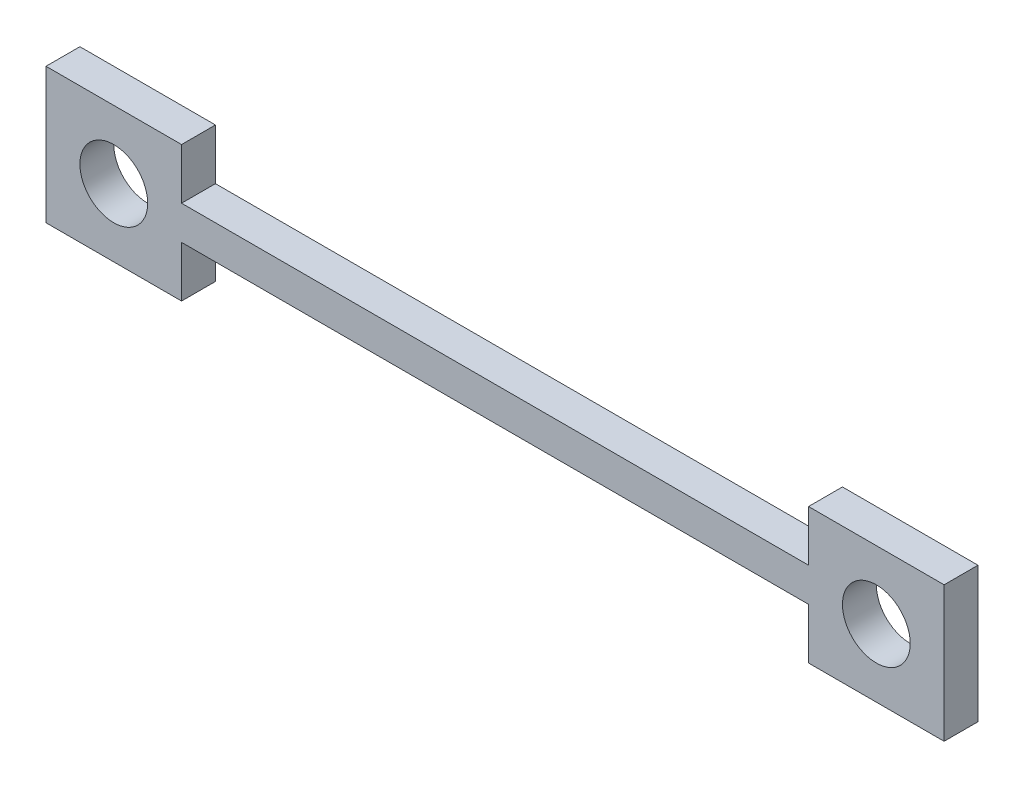
from build123d import *

# Parameters (mm, degrees)
SKETCH1_R           = 100
BOSS_EXTRUDE1_DEPTH = 100


with BuildPart() as part:
    # Sketch1 → Boss-Extrude1 (new body)
    with BuildSketch(Plane.XY):
        Polygon((200, 50), (2050, 50), (2050, 200), (2450, 200), (2450, -200), (2050, -200), (2050, -50), (200, -50), (200, -200), (-200, -200), (-200, 200), (200, 200), align=None)
        Circle(SKETCH1_R, mode=Mode.SUBTRACT)
        with Locations((2250, 0)):
            Circle(SKETCH1_R, mode=Mode.SUBTRACT)
    extrude(amount=BOSS_EXTRUDE1_DEPTH)


solid = part.part
